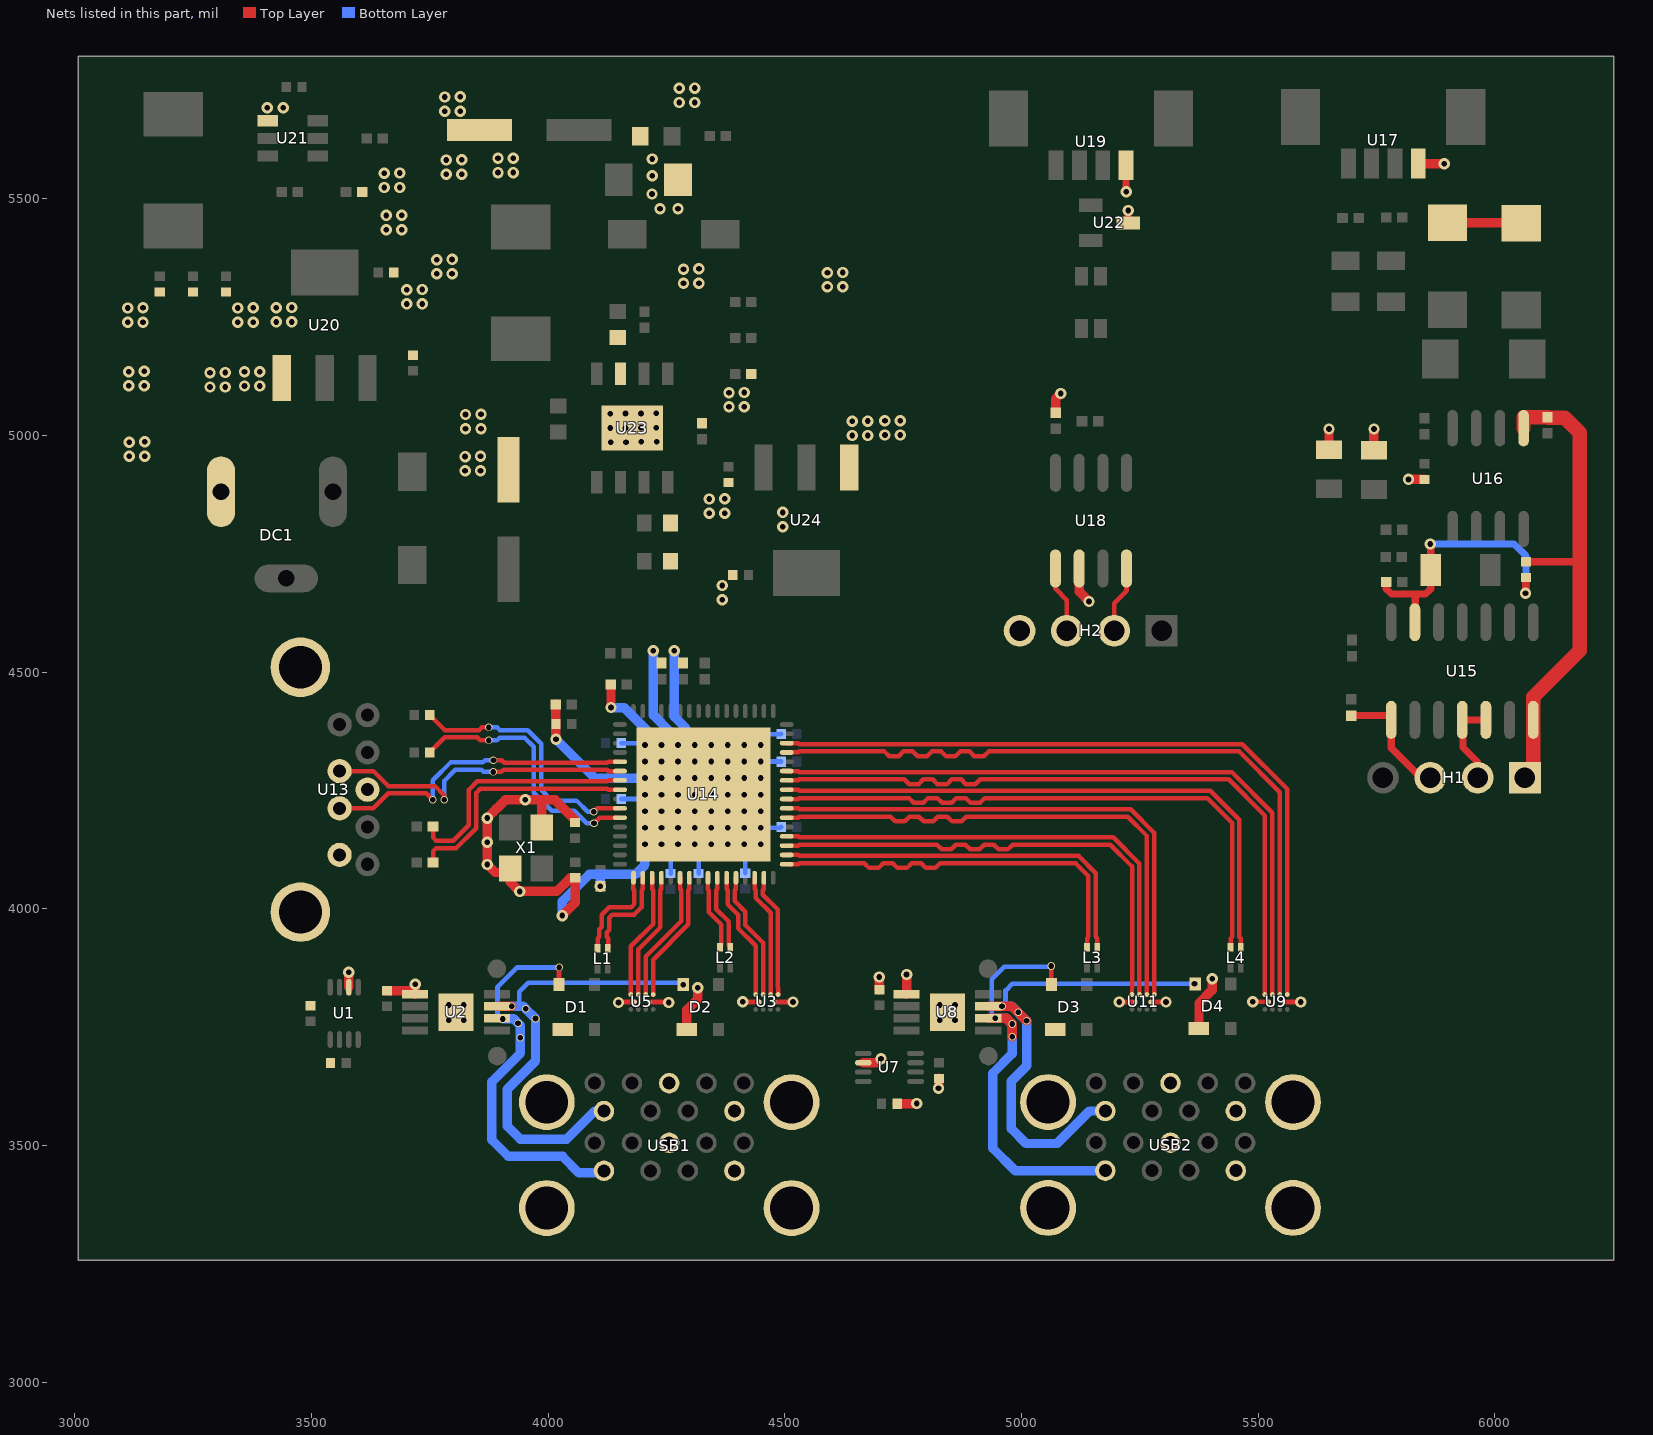
[diagram p0: the nets of this part, all layers, seen from the top]
# Altium PCB MISC51972.pcbdoc (part 3 of 3)
Units mil, origin at the board's own origin, x right, y up, seen from the top; angles counter-clockwise.
Board outline 3243 x 2543 mil, 4 copper layers (Top Layer, GND, Signal-1, Bottom Layer), stack 62.447 mil thick; 117 components, 123 nets, 473 pads, 324 vias.

## Via types
v1: diameter 24.02, hole 12, Top Layer to Bottom Layer, 276 vias
v2: diameter 16, hole 12, Top Layer to Bottom Layer, 47 vias
v3: diameter 24, hole 16, Top Layer to Bottom Layer, 1 vias

## Nets (pads, with @x,y where several pads share a name; then routed paths per layer and width w, separated by ;. In a path a pad name is that pad's centre, name@x,y a point inside that pad or via, vN(x,y) a via of type N, cw(c..) or ccw(c..) an arc to the next point about the centre after c; other vN are vias at no path point) (continued)
GND: C1.1 C2.2 C3.2 C4.1 C5.2 C6.2 C9.1 C10.1 C11.1 C12.1 C13.1 C14.1 C15.2 C16.1 C17.2 C18.1 C19.1 C20.1 C21.1 C23.1 C24.1 C25.1 C27.1 C28.1 C30.1 C31.2 C32.2 C33.1 C34.1 C35.1 C36.1 C37.2 D1.1 D2.1 D3.1 D4.1 DC1.2 H1.1 H2.4 LED1.2 R3.2 R9.2 R11.2 R12.2 R13.2 R16.1 R19.2 R23.2 R27.1 R28.2 RXD1.2 TXD1.2 U1.2 U2.1 U2.9 U3.B1 U3.B2 U5.B1 U5.B2 U7.2 U8.1 U8.9 U9.B1 U9.B2 U11.B1 U11.B2 U13.4 U13.7 U13.10 U14.65 U15.7 U16.5 U17.1 U18.2 U19.1 U20.1 U21.1 U22.3 U23.7 U23.9 U24.1 USB1.4 USB1.7 USB1.13 USB1.16 USB1.19 USB1.20 USB2.4 USB2.7 USB2.13 USB2.16 USB2.19 USB2.20 X1.2 X1.4 | length 4533.2
  Top Layer w10: v1(4148.5,3802.5) 4149.51,3803.51 U5.B1@4182.25,3803.51 ; U5.B2@4213.75,3803.51 4253.49,3803.51 v1(4254.5,3802.5) ; v1(4411,3804) 4411.49,3803.51 U3.B1@4446,3803.51 ; U3.B2@4477.5,3803.51 v1(4517,3803.51) ; v1(5206,3803.51) U11.B1@5241.1,3803.51 ; U11.B2@5272.6,3803.51 v1(5305,3803.51) ; v1(5488.5,3804) 5521.46,3804 U9.B1@5521.95,3803.51 ; U9.B2@5553.45,3803.51 v1(5590,3803.51)
  Top Layer w15: U19.1@5220.66,5571.14 5220.66,5515.34 v1(5221,5515) ; U22.3@5225.01,5449.36 v1(5225,5475.5) ; C21.1@6065.5,4733.54 6178.84,4733.54 6179.1,4733.8
  Top Layer w20: U1.2@3578.64,3834.62 v1(3578.64,3866) ; C2.2@3659.5,3827.54 3710.94,3827.54 U2.1@3718.49,3819.99 3718.49,3840.49 v1(3719,3841) ; X1.2@3986.47,4172.51 3986.47,4228.63 3988.34,4230.5 ; R11.2@4015.76,4432.4 4016.26,4431.9 C17.2@4016.26,4390.72 v1(4016.26,4358.5) ; v1(4029.5,3986) 4057,4013.5 C9.1@4057,4065.76 4046.76,4065.76 4018,4037 v1(3939.5,4037) 3919.53,4056.97 X1.4@3919.53,4085.89 3910.64,4077 3888,4077 v1(3871,4094) v1(3871,4140.97) v1(3871,4192) 3883.63,4204.63 3883.63,4205.16 3890.82,4212.35 3891.35,4212.35 3909.5,4230.5 v1(3951.53,4230.5) 3988.34,4230.5 ; C10.1@4056.7,4182.64 4056.7,4188.3 4014.5,4230.5 3988.34,4230.5 ; R9.2@4132.12,4473.9 4132.5,4473.52 v1(4132.5,4425.5) ; D2.1@4292.87,3745.56 4292.87,3786.87 4316,3810 v1(4316,3833.5) ; U7.2@4665.55,3675.12 4694.62,3675.12 v1(4703,3683.5) ; C5.2@4699.5,3829.54 v1@4699.5,3856.23 ; C6.2@4737.04,3588.5 4778,3588.5 v1(4778.5,3589) ; U8.1@4756.39,3819.99 4756.98,3820.58 v1(4756.98,3861.62) ; v1(4824.5,3621.5) 4825.5,3622.5 C4.1@4825.5,3641.96 ; R19.2@5072.14,5048.44 5072.14,5078.14 v1(5083,5089) ; U18.2@5121.64,4719.18 5121.64,4670.36 v1(5142.5,4649.5) ; D4.1@5374.77,3747.06 5374.77,3800.77 5402.5,3828.5 v1(5402.5,3852.5) ; TXD1.2@5649.45,4970.52 v1(5649.45,5014) ; RXD1.2@5744.45,4969.02 v1(5744.45,5014) ; v1(5817.5,4907.46) C15.2@5851,4907.46 ; U17.1@5837.97,5574.64 v1(5893,5574.64)
  Top Layer w30: U16.5@6060.45,5015.66 6060.45,5038.66 R16.1@6111.45,5038.66 6112.51,5037.6 6147.6,5037.6 6179.1,5006.1 6179.1,4733.8 6179.1,4546.1 6080.95,4447.95 U15.7@6080.95,4399.55 6080.95,4294.95 H1.1@6063.5,4277.5
  Bottom Layer w10: C12.1@4153.94,4232.3 4195.01,4232.3 v1(4204.21,4241.5) ; C20.1@4153.94,4350.3 4200.41,4350.3 v1(4204.21,4346.5) ; C11.1@4258.6,4075.04 4258.6,4120.89 v1(4274.21,4136.5) ; v1(4309.21,4136.5) 4317.8,4127.91 C19.1@4317.8,4075.04 ; v1(4414.21,4136.5) 4416.1,4134.61 C13.1@4416.1,4075.74 ; v1(4449.21,4171.5) 4490.32,4171.5 C14.1@4492.02,4173.2 ; v1(4449.21,4311.5) 4491.52,4311.5 C18.1@4492.02,4311 ; v1(4449.21,4346.5) 4449.21,4362.49 4455.92,4369.21 4491.13,4369.21 C16.1@4492.02,4370.1
  Bottom Layer w20: v1(4016.26,4358.5) 4098.26,4276.5 v1(4204.21,4276.5) ; v1(4029.5,3986) 4029.5,4016 4086.5,4073 4107.62,4073 ; v1(4110,4047.96) 4110,4070.62 4107.62,4073 ; v1(4132.5,4425.5) 4160.21,4425.5 v1(4239.21,4346.5) ; v1(4204.21,4136.5) 4204.21,4093.21 4184,4073 4107.62,4073 ; v1(4222,4545.5) 4222,4409.5 4256.5,4375 ; v1(4266.22,4545.5) 4266.22,4406.28 4290.5,4382
  other v1: 3789.5,3765 3821.5,3765 4827.4,3765 4859.4,3765 3789.5,3797 3821.5,3797 4827.4,3797 4859.4,3797 4699.46,3856.27 4239.21,4136.5 4344.21,4136.5 4379.21,4136.5 4449.21,4136.5 4204.21,4171.5 4239.21,4171.5 4274.21,4171.5 4309.21,4171.5 4344.21,4171.5 4379.21,4171.5 4414.21,4171.5 4204.21,4206.5 4239.21,4206.5 4274.21,4206.5 4309.21,4206.5 4344.21,4206.5 4379.21,4206.5 4414.21,4206.5 4449.21,4206.5 4239.21,4241.5 4274.21,4241.5 4309.21,4241.5 4344.21,4241.5 4379.21,4241.5 4414.21,4241.5 4449.21,4241.5 4239.21,4276.5 4274.21,4276.5 4309.21,4276.5 4344.21,4276.5 4379.21,4276.5 4414.21,4276.5 4449.21,4276.5 4204.21,4311.5 4239.21,4311.5 4274.21,4311.5 4309.21,4311.5 4344.21,4311.5 4379.21,4311.5 4414.21,4311.5 4274.21,4346.5 4309.21,4346.5 4344.21,4346.5 4379.21,4346.5 4414.21,4346.5 4367.25,4653.25 4367.25,4683.25 4495.25,4807.75 4340.25,4836.25 4372.75,4836.25 4495.25,4837.75 4340.25,4866.25 4372.75,4866.75 3824.25,4925.75 3856.75,4925.75 3114.75,4956.25 3147.25,4956.25 3824.25,4955.75 3856.75,4956.25 3114.75,4986.25 4131.75,4986.25 4164.25,4986.25 3147.25,4986.75 4196.75,4986.75 4229.25,4986.75 4642.25,5000.25 4674.75,5000.25 4711.25,5001.25 4743.75,5001.25 3825.25,5014.75 3857.75,5014.75 4130.75,5016.25 4163.25,5016.25 4195.75,5016.75 4228.25,5016.75 4642.25,5030.25 4674.75,5030.75 4711.25,5031.25 4743.75,5031.75 3825.25,5044.75 3857.75,5045.25 4130.75,5046.25 4163.25,5046.75 4195.75,5046.75 4228.25,5047.25 4381.75,5060.75 4414.25,5060.75 4381.75,5090.75 4414.25,5091.25 3285.25,5102.75 3317.75,5102.75 3113.75,5105.25 3146.25,5105.25 3358.25,5104.75 3390.75,5104.75 3285.25,5132.75 3317.75,5133.25 3113.75,5135.25 3358.25,5134.75 3390.75,5135.25 3146.25,5135.75 3111.25,5239.75 3143.75,5239.75 3344.25,5239.75 3376.75,5239.75 3425.25,5240.25 3457.75,5240.25 3111.25,5269.75 3143.75,5270.25 3344.25,5269.75 3376.75,5270.25 3425.25,5270.25 3457.75,5270.75 3701.25,5278.25 3733.75,5278.25 3701.25,5308.25 3733.75,5308.75 4589.75,5314.25 4622.25,5314.25 4285.75,5321.75 4318.25,5321.75 3764.25,5341.75 3796.75,5341.75 4589.75,5344.25 4622.25,5344.75 4285.75,5351.75 4318.25,5352.25 3764.25,5371.75 3796.75,5372.25 3657.75,5435.25 3690.25,5435.25 3657.75,5465.25 3690.25,5465.75 4235.91,5478.99 4274.2,5478.99 4219,5510.5 3653.75,5524.25 3686.25,5524.25 4219.5,5549 3784.75,5552.25 3817.25,5552.25 3653.75,5554.25 3686.25,5554.75 3893.75,5555.75 3926.25,5555.75 3784.75,5582.25 3817.25,5582.75 4219.5,5584.5 3893.75,5585.75 3926.25,5586.25 3781.5,5685.5 3814,5685.5 3406.51,5693 3439.87,5693 4276.75,5703.75 4309.25,5703.75 3781.5,5715.5 3814,5716 4276.75,5733.75 4309.25,5734.25
GND485: D5.2 D7.1 | length 156.2
  Top Layer w20: D7.1@5899.45,5449.39 6054.95,5449.39 D5.2@6055.45,5448.89
P74_TXD6: H1.3 R5.1 U15.1 | length 256.4
  Top Layer w15: R5.1@5696.45,4408.62 5771.88,4408.62 U15.1@5780.95,4399.55 5780.95,4339.75 5843.2,4277.5 H1.3@5863.5,4277.5
P75_RXD6: H1.2 U15.4 U15.5 | length 185.5
  Top Layer w15: H1.2@5963.5,4277.5 5963.5,4310.2 5932.6,4341.1 5932.6,4397.9 U15.4@5930.95,4399.55 U15.5@5980.95,4399.55
P84_CAN_TX2: H2.3 U18.1 | length 141.3
  Top Layer w10: U18.1@5071.64,4719.18 5071.64,4676.36 5095.5,4652.5 5095.5,4588 H2.3@5095.64,4587.86
P85_CAN_RX2: H2.2 U18.4 | length 142.2
  Top Layer w10: H2.2@5195.64,4587.86 5195.5,4588 5195.5,4646 5221.64,4672.14 U18.4@5221.64,4719.18
R5+: C21.2 D8.2 R15.2 U15.13 | length 599.3
  Top Layer w15: R15.2@5770.45,4691.16 5770.45,4676.25 5781.6,4665.1 5831.6,4665.1 ; U15.13@5830.95,4605.77 5831.6,4606.42 5831.6,4665.1 ; v1(5863.1,4771.1) 5864.46,4769.74 D8.2@5864.46,4716.16 5864.46,4675.96 5853.6,4665.1 5831.6,4665.1 ; v1(6064.6,4667.1) 6064.6,4699.56 C21.2@6065.5,4700.46
  Bottom Layer w15: v1(5863.1,4771.1) 6040.6,4771.1 6065.6,4746.1 6065.6,4668.1 v1(6064.6,4667.1)
USB5_5V: D2.4 U2.7 USB1.10 | length 973.4
  Top Layer w20: U2.7@3891.71,3794.4 3891.81,3794.5 v2(3922.5,3794.5)
  Bottom Layer w10: 3936.65,3794.5 3938.5,3796.35 3938.5,3825 3957.5,3844 4281.04,3844 v2(4285,3840.04)
  Bottom Layer w20: v2(3922.5,3794.5) 3936.65,3794.5 3947.5,3794.5 3952.42,3789.58 v2(3952.42,3788.99) v2(3973,3768.41) 3973,3679 3913.5,3619.5 3913.5,3541 3941,3513.5 4038.5,3513.5 4098.13,3573.13 USB1.10@4119,3573.13
USB6_5V: D1.4 U2.6 USB1.1 | length 835.3
  Top Layer w10: D1.4@4022.6,3840.04 4022.6,3876.1 v2(4023,3876.5)
  Bottom Layer w10: v2(3903.5,3767.58) 3892.5,3778.58 3892.5,3834.5 3934.5,3876.5 v2(4023,3876.5)
  Bottom Layer w20: v2(3903.5,3767.58) 3927.28,3767.58 v2(3936.18,3758.68) 3940.68,3754.18 v2(3940.68,3727.99) 3940.68,3694.68 3880.5,3634.5 3880.5,3512.5 3915.5,3477.5 4030.5,3477.5 4030.5,3476.5 4064.5,3442.5 4114.35,3442.5 USB1.1@4119,3447.15
USB7_5V: D4.4 U8.7 USB2.10 | length 1081.4
  Top Layer w20: U8.7@4929.61,3794.4 v2(4958.65,3794.4) 4979.1,3794.4 4991.61,3781.89 v2(4993.11,3781.89) 4993.11,3780.89 v2(5010.5,3763.5)
  Bottom Layer w10: v2(4958.65,3794.4) 4966,3801.75 4966,3827.5 4980.54,3842.04 v2(5365.4,3842.04)
  Bottom Layer w20: v2(4958.65,3794.4) 4979.6,3794.4 v2(5010.5,3763.5) 5010.5,3668.5 4978.5,3636.5 4978.5,3535.5 5009.5,3504.5 5075,3504.5 5143.63,3573.13 USB2.10@5176.88,3573.13
USB8_5V: D3.4 U8.6 USB2.1 | length 922.5
  Top Layer w10: D3.4@5062.9,3840.04 v2(5062.9,3879.5)
  Top Layer w20: U8.6@4929.61,3768.8 v2(4944.33,3768.8) 4968.2,3768.8 v2(4980,3757) v2(4980,3730)
  Bottom Layer w10: v2(4944.33,3768.8) 4937,3776.13 4937,3851.5 4963.5,3878 5061.4,3878 v2(5062.9,3879.5)
  Bottom Layer w20: v2(4944.33,3768.8) 4968.2,3768.8 v2(4980,3757) v2(4980,3730) 4980,3694 4939,3653 4939,3494.5 4986.35,3447.15 USB2.1@5176.88,3447.15
USB30_SSRXM: R2.2 U14.56 | length 517.9
  Top Layer w9.5: R2.2@3756.49,4098.28 3756.49,4121.92 3763.21,4128.63 3805.92,4128.63 3847.5,4170.21 3847.5,4245 3856.53,4254.03 4125.05,4254.03 4127.15,4251.94 U14.56@4151.41,4251.94
USB30_SSRXP: R1.2 U14.55 | length 517.9
  Top Layer w9.5: R1.2@3756.49,4174.48 3756.49,4150.85 3763.21,4144.13 3799.5,4144.13 3832,4176.63 3832,4251.42 3850.11,4269.53 4125.05,4269.53 4127.15,4271.63 U14.55@4151.41,4271.63
USB30_SSTXM: C8.2 U14.59 | length 556.7
  Top Layer w9.5: C8.2@3749.79,4330.78 3781.49,4362.48 3850.1,4362.48 3856.5,4356.09 v2(3874,4356.09) ; v2(4096.63,4181.02) 4108.61,4193 4151.3,4193 U14.59@4151.41,4192.89
  Bottom Layer w9.5: v2(3874,4356.09) 3891.5,4356.09 3897.46,4362.04 3949.96,4362.04 3969.5,4342.5 3969.5,4245.5 4007.5,4207.5 4055.03,4207.5 4081.5,4181.02 v2(4096.63,4181.02)
USB30_SSTXP: C7.2 U14.58 | length 550.8
  Top Layer w9.5: C7.2@3749.79,4409.68 3781.49,4377.98 3853.98,4377.98 3859.5,4383.5 v2(3874.5,4383.5) ; v2(4096.13,4205.16) 4103.54,4212.57 U14.58@4151.41,4212.57
  Bottom Layer w9.5: v2(3874.5,4383.5) 3892,4383.5 3897.96,4377.54 3956.38,4377.54 3985,4348.92 3985,4251.92 4007.92,4229 4059.5,4229 4083.34,4205.16 v2(4096.13,4205.16)
USB30_T_DM1: L1.1 U14.2 | length 206.8
  Top Layer w9.5: L1.1@4126.43,3919.05 4126.43,3937.7 4123.35,3940.78 4123.35,3950.28 4128.78,3955.72 4128.78,3981.57 4135.5,3988.28 4181.75,3988.28 4197.55,4004.08 4197.55,4039.56 4199.64,4041.66 U14.2@4199.64,4065.92
USB30_T_DM2: L2.1 U14.10 | length 159.9
  Top Layer w9.5: U14.10@4357.12,4065.92 4357.12,4041.66 4355.02,4039.56 4355.02,3999.4 4381,3973.42 4381,3922.38 L2.1@4384.33,3919.05
USB30_T_DM3: L3.1 U14.18 | length 826.9
  Top Layer w9.5: U14.18@4503.77,4114.15 4528.03,4114.15 4530.13,4112.06 5120.44,4112.06 5156.75,4075.75 5156.75,3940.78 5159.83,3937.7 L3.1@5159.83,3919.05
USB30_T_DM4: L4.1 U14.25 | length 1253.3
  Top Layer w9.5: U14.25@4503.77,4251.94 4528.03,4251.94 4530.12,4249.85 5398.72,4249.85 5460.15,4188.42 5460.15,3940.78 5463.23,3937.7 L4.1@5463.23,3919.05
USB30_T_DP1: L1.4 U14.1 | length 206.8
  Top Layer w9.5: L1.4@4104.77,3919.05 4104.77,3937.7 4107.85,3940.78 4107.85,3956.7 4113.28,3962.14 4113.28,3987.99 4129.08,4003.78 4175.33,4003.78 4182.05,4010.5 4182.05,4039.56 4179.95,4041.66 U14.1@4179.95,4065.92
USB30_T_DP2: L2.4 U14.9 | length 159.7
  Top Layer w9.5: U14.9@4337.43,4065.92 4337.43,4041.66 4339.52,4039.56 4339.52,3992.97 4365.5,3967 4365.5,3921.88 L2.4@4362.67,3919.05
USB30_T_DP3: L3.4 U14.17 | length 826
  Top Layer w9.5: U14.17@4503.77,4094.46 4528.03,4094.46 4530.13,4096.56 4667.71,4096.56 4677.71,4086.55 4697.71,4086.55 4707.71,4096.56 4727.71,4096.56 4737.71,4086.55 4757.71,4086.55 4767.71,4096.56 4787.71,4096.56 4797.71,4086.55 4817.71,4086.55 4827.71,4096.56 5114.02,4096.56 5141.25,4069.33 5141.25,3940.78 5138.17,3937.7 L3.4@5138.17,3919.05
USB30_T_DP4: L4.4 U14.24 | length 1252.5
  Top Layer w9.5: U14.24@4503.77,4232.26 4528.03,4232.26 4530.12,4234.35 4762.11,4234.35 4772.11,4224.35 4792.11,4224.35 4802.11,4234.35 4822.11,4234.35 4832.11,4224.35 4852.11,4224.35 4862.11,4234.35 4882.11,4234.35 4892.11,4224.35 4912.11,4224.35 4922.11,4234.35 5392.3,4234.35 5444.65,4182 5444.65,3940.78 5441.57,3937.7 L4.4@5441.57,3919.05
USB30_T_SSRXM1: U5.A4 U14.7 | length 278.4
  Top Layer w9.5: U5.A4@4221.62,3819.26 4221.62,3833.76 4221.49,3833.89 4221.49,3892.99 4295.97,3967.47 4295.97,4039.57 4298.06,4041.66 U14.7@4298.06,4065.92
USB30_T_SSRXM2: U3.A4 U14.15 | length 260.7
  Top Layer w9.5: U14.15@4455.54,4065.92 4455.54,4041.66 4453.45,4039.57 4453.45,4030.07 4485.24,3998.27 4485.24,3833.89 4485.37,3833.76 U3.A4@4485.37,3819.26
USB30_T_SSRXM3: U11.A4 U14.23 | length 1139.5
  Top Layer w9.5: U14.23@4503.77,4212.57 4528.03,4212.57 4530.12,4210.48 5230.52,4210.48 5280.35,4160.65 5280.35,3833.89 5280.47,3833.76 U11.A4@5280.47,3819.26
USB30_T_SSRXM4: U9.A4 U14.30 | length 1541
  Top Layer w9.5: U9.A4@5561.32,3819.26 5561.32,3833.76 5561.19,3833.89 5561.19,4253.31 5466.23,4348.27 4530.13,4348.27 4528.03,4350.37 U14.30@4510.19,4350.37 ; U14.30@4510.19,4350.37 U14.30@4503.77,4350.37 4504.8,4349.34 4511.22,4349.34 U14.30@4510.19,4350.37
USB30_T_SSRXP1: U5.A3 U14.6 | length 278.4
  Top Layer w9.5: U5.A3@4205.87,3819.26 4205.87,3833.76 4205.99,3833.89 4205.99,3899.42 4280.47,3973.89 4280.47,4039.57 4278.38,4041.66 U14.6@4278.38,4065.92
USB30_T_SSRXP2: U3.A3 U14.14 | length 260.7
  Top Layer w9.5: U14.14@4435.86,4065.92 4435.86,4041.66 4437.95,4039.57 4437.95,4023.65 4469.74,3991.85 4469.74,3833.89 4469.62,3833.76 U3.A3@4469.62,3819.26
USB30_T_SSRXP3: U11.A3 U14.22 | length 1138.7
  Top Layer w9.5: U14.22@4503.77,4192.89 4528.03,4192.89 4530.12,4194.98 4723.03,4194.98 4733.03,4184.98 4753.03,4184.98 4763.03,4194.98 4783.03,4194.98 4793.03,4184.98 4813.03,4184.98 4823.03,4194.98 4843.03,4194.98 4853.03,4184.98 4873.03,4184.98 4883.03,4194.98 5224.1,4194.98 5264.85,4154.23 5264.85,3833.89 5264.72,3833.76 U11.A3@5264.72,3819.26
USB30_T_SSRXP4: U9.A3 U14.29 | length 1539.2
  Top Layer w9.5: U14.29@4503.77,4330.68 4528.03,4330.68 4530.13,4332.77 4710.28,4332.77 4720.28,4322.77 4740.28,4322.77 4750.28,4332.77 4770.28,4332.77 4780.28,4322.77 4800.28,4322.77 4810.28,4332.77 4830.28,4332.77 4840.28,4322.77 4860.28,4322.77 4870.28,4332.77 4890.28,4332.77 4900.28,4322.77 4920.28,4322.77 4930.28,4332.77 5459.8,4332.77 5545.69,4246.88 5545.69,3833.89 5545.57,3833.76 U9.A3@5545.57,3819.26
USB30_T_SSTXM1: U5.A2 U14.4 | length 267
  Top Layer w9.5: 4189.96,3849.85 4189.96,3914.54 4236.91,3961.49 4236.91,4039.56 4239.01,4041.66 U14.4@4239.01,4065.92 ; 4190.01,3849.81 4190.01,3833.89 4190.13,3833.76 U5.A2@4190.13,3819.26
USB30_T_SSTXM2: U3.A2 U14.12 | length 272.2
  Top Layer w9.5: U14.12@4396.49,4065.92 4396.49,4041.66 4394.4,4039.56 4394.4,4016 4416.49,3993.91 4416.49,3966 4453.76,3928.73 4453.76,3833.89 4453.88,3833.76 U3.A2@4453.88,3819.26
USB30_T_SSTXM3: U11.A2 U14.20 | length 1045.8
  Top Layer w9.5: U14.20@4503.77,4153.52 4528.03,4153.52 4530.13,4151.43 5193.57,4151.43 5248.85,4096.15 5248.85,3833.89 5248.98,3833.76 U11.A2@5248.98,3819.26
USB30_T_SSTXM4: U9.A2 U14.27 | length 1446.5
  Top Layer w9.5: U14.27@4503.77,4291.31 4528.03,4291.31 4530.12,4289.22 5443.78,4289.22 5529.7,4203.3 5529.7,3833.89 5529.83,3833.76 U9.A2@5529.83,3819.26
USB30_T_SSTXP1: U5.A1 U14.3 | length 267
  Top Layer w9.5: U5.A1@4174.38,3819.26 4174.38,3833.76 4174.51,3833.89 4174.51,3849.81 ; 4174.46,3849.85 4174.46,3920.96 4221.41,3967.91 4221.41,4039.56 4219.32,4041.66 U14.3@4219.32,4065.92
USB30_T_SSTXP2: U3.A1 U14.11 | length 272.2
  Top Layer w9.5: U14.11@4376.8,4065.92 4376.8,4041.66 4378.9,4039.56 4378.9,4009.58 4400.99,3987.49 4400.99,3959.58 4438.26,3922.31 4438.26,3833.89 4438.13,3833.76 U3.A1@4438.13,3819.26
USB30_T_SSTXP3: U11.A1 U14.19 | length 1045
  Top Layer w9.5: U14.19@4503.77,4133.83 4528.03,4133.83 4530.13,4135.93 4821.21,4135.93 4831.21,4125.93 4851.21,4125.93 4861.21,4135.93 4881.21,4135.93 4891.21,4125.93 4911.21,4125.93 4921.21,4135.93 4941.21,4135.93 4951.21,4125.93 4971.21,4125.93 4981.21,4135.93 5187.15,4135.93 5233.35,4089.72 5233.35,3833.89 5233.23,3833.76 U11.A1@5233.23,3819.26
USB30_T_SSTXP4: U9.A1 U14.26 | length 1445.6
  Top Layer w9.5: U14.26@4503.77,4271.63 4528.03,4271.63 4530.12,4273.72 4752.29,4273.72 4762.29,4263.72 4782.29,4263.72 4792.29,4273.72 4812.29,4273.72 4822.29,4263.72 4842.29,4263.72 4852.29,4273.72 4872.29,4273.72 4882.29,4263.72 4902.29,4263.72 4912.29,4273.72 5437.36,4273.72 5514.2,4196.87 5514.2,3833.89 5514.08,3833.76 U9.A1@5514.08,3819.26
USB30_USB_DM: U13.2 U14.54 | length 677.3
  Top Layer w9.5: U13.2@3559.07,4291.36 3630.12,4291.35 3661.74,4259.73 3760.54,4259.73 3780.03,4240.25 v2(3780.03,4230.83) ; v2(3883.5,4289.5) 3901,4289.5 3905.6,4294.1 4124.36,4294.1 4127.15,4291.31 U14.54@4151.41,4291.31
  Bottom Layer w9.5: v2(3780.03,4230.83) 3780.03,4270.35 3803.77,4294.1 3858.4,4294.1 3863,4289.5 v2(3883.5,4289.5)
USB30_USB_DP: U13.3 U14.53 | length 673.3
  Top Layer w9.5: U13.3@3559.07,4212.62 3630.12,4212.61 3661.74,4244.23 3742.38,4244.23 v2(3756.04,4230.57) ; v2(3884.1,4314.19) 3901.6,4314.19 3907.19,4308.6 4124.74,4308.6 4127.15,4311 U14.53@4151.41,4311
  Bottom Layer w9.5: v2(3756.04,4230.57) 3756.04,4272.04 3793.6,4309.6 3862,4309.6 3866.6,4314.19 v2(3884.1,4314.19)
pads on no net: DC1.3 U14.32 U14.33 U14.35 U14.36 U14.37 U14.38 U14.39 U14.41 U14.43 U14.44 U14.46 U14.47 U14.60 U17.5 U17.6 U18.5 U19.5 U19.6

## Polygon pours and split planes (outlines as drawn)
1.8V on Signal-1 (solid, remove dead copper): 3443.5,5314 3443.5,5480.29 3416.72,5507.06 3261.56,5507.06 3226.5,5472 3226.5,3916 3374,3768.5 4918,3768.5 4918,3313 4885.5,3280.5 3183.5,3280.5 3060.5,3403.5 3060.5,5517 3167.5,5624 3603,5624 3613,5614 3613,5302.54 3589.7,5279.24 3478.26,5279.24
GND on Top Layer (solid, remove dead copper, pour order 26): 4768,4454 3622,4454 3622,3281.5 3017.5,3281.5 3017.5,4454 3003.25,4454 3003.25,5801 4768,5801
GND on Bottom Layer (solid, remove dead copper, pour order 32): 4765,4453 3632.5,4453 3632.5,3271.5 3000,3271.5 3000,4453 3007.5,4453 3007.5,5801 4765,5801
D5.0V on Signal-1 (solid, remove dead copper): 4894.5,3913.19 4781.31,3800 3350,3800 3233,3917 3233,4362.5 3296.5,4426 3576,4426 3584.5,4417.5 3584.5,4365 3570.5,4351 3399.5,4351 3357.5,4309 3357.5,3982 3407.5,3932 4625,3932 4675.5,3982.5 4675.5,4725.5 4631.5,4769.5 4373,4769.5 4313.5,4829 4313.5,5616.54 4349.29,5652.33 4520.67,5652.33 4547,5626 4547,4961 4587,4921 4866,4921 4894.5,4892.5
12V on Top Layer (solid, remove dead copper, pour order 0): 3495,4963.5 3548,5016.5 3575.5,5016.5 3583.5,5024.5 3583.5,5166.38 3596.13,5179.01 3654.49,5179.01 3679,5154.5 3747,5154.5 3759.5,5142 3759.5,4877 3746,4863.5 3629.5,4863.5 3614.5,4848.5 3614.5,4790.5 3600.5,4776.5 3519.5,4776.5 3495,4801
$1N10192 on Top Layer (solid, remove dead copper, pour order 2): 3671,4798.5 4102,4798.5 4132,4828.5 4132,4927.66 4139.53,4935.19 4214.31,4935.19 4220.5,4929 4220.5,4662.57 4203.62,4645.69 3666.81,4645.69 3641.5,4671 3641.5,4775.5 3665,4799 3670.5,4799
$1N10194 on Top Layer (solid, remove dead copper, pour order 4): 3841,5251 4102.98,5251 4116.78,5237.2 4116.78,5106.75 4114.03,5103 4047,5103 4042,5098 4042,5047.17 4037.07,5042.23 3962.27,5042.23 3954.5,5050 3954.5,5093 3945,5102.5 3836,5102.5 3824.5,5114 3824.5,5234.5
$1N10186 on Top Layer (solid, remove dead copper, pour order 6): 3996.5,5679.5 4131,5679.5 4138,5672.5 4138,5591.32 4145.8,5583.52 4179.98,5583.52 4182.5,5581 4182.5,5464 4185.5,5461 4211,5461 4214.5,5457.5 4214.5,5393 4210,5388.5 3877,5388.5 3870.5,5395 3870.5,5487 3877,5493.5 3978.5,5493.5 3987,5502 3987,5670
D5.0V on Top Layer (solid, remove dead copper, pour order 8): 4371,5659 4362.5,5650.5 4362.5,5475 4353.5,5466 4314,5466 4307.5,5459.5 4307.5,5390.5 4322,5376 4364.5,5376 4373.5,5367 4373.5,5271.59 4382.12,5262.97 4397.97,5262.97 4407,5272 4407,5303 4417.5,5313.5 4454.5,5313.5 4475.5,5334.5 4475.5,5652.5 4468.5,5659.5 4468,5659
1.1V on Top Layer (solid, remove dead copper, pour order 10): 3147,5494.5 3344.5,5494.5 3356.5,5482.5 3356.5,5336.99 3343.91,5324.4 3148.1,5324.4 3137.5,5335 3137.5,5485
1.1V on Signal-1 (solid, remove dead copper): 3259,5484 3349.99,5484 3383.49,5450.5 3383.49,5166.51 3434.5,5115.5 4045,5115.5 4088,5072.5 4088,4090 4126.5,4051.5 4515,4051.5 4553.5,4090 4553.5,4390.5 4570.5,4407.5 4654.5,4407.5 4671.5,4390.5 4671.5,3990.5 4618.5,3937.5 4029.5,3937.5 3921.5,4045.5 3921.5,4903 3839.5,4985 3286.04,4985 3235.81,5035.22 3235.81,5460.81
3.3V on Top Layer (solid, remove dead copper, pour order 12): 4593,5188.5 4593,5064.5 4757.5,5064.5 4757.5,5188.5
1.8V on Top Layer (solid, remove dead copper, pour order 14): 3489,5152 3489,5028.5 3561.5,5028.5 3561.5,5152
GND on Bottom Layer (solid, remove dead copper, pour order 28): 4185.5,4384 4185.5,4100 4469.5,4100 4469.5,4384
GND on Bottom Layer (solid, remove dead copper, pour order 30): 4185.5,4384 4185.5,4100 4469.5,4100 4469.5,4384
GND on Signal-1 (solid, remove dead copper): 4185.5,4384 4185.5,4100 4469.5,4100 4469.5,4384
3.3V on Signal-1 (solid, remove dead copper): 4483.5,4403 4170.5,4403 4170.5,4105 4113,4105 4113,4580.5 4165,4632.5 4438,4632.5 4460,4654.5 4460,4749.23 4471.77,4761 4620,4761 4629,4752 4629,4426.5 4617,4414.5 4538,4414.5 4538,4084.5 4483.5,4084.5
D5.0V on Top Layer (solid, remove dead copper, pour order 16): 3744.8,3806 3748.52,3802.28 3748.52,3788.02 3744,3783.5 3599,3783.5 3584.5,3769 3584.5,3709 3580.5,3705 3557.5,3705 3552,3710.5 3552,3790.5 3567.5,3806
1.8V on Top Layer (solid, remove dead copper, pour order 18): 3482.27,3770.58 3482.27,3702.5 3544,3702.5 3544,3770.58
1.8V on Top Layer (solid, remove dead copper, pour order 20): 4643.5,3661.5 4643.5,3574.7 4713,3574.7 4713,3661.5
D5.0V on Top Layer (solid, remove dead copper, pour order 22): 4756.5,3684 4808.93,3684 4811.83,3686.9 4837.57,3686.9 4841.33,3683.14 4841.33,3665.33 4838,3662 4800.17,3662 4796.67,3658.5 4796.67,3650.67 4793,3647 4757,3647 4752.5,3651.5 4752.5,3680
D5.0V on Top Layer (solid, remove dead copper, pour order 24): 4603.5,3860.5 4603.5,3796.46 4665.93,3796.46 4665.93,3860.5
GND on Bottom Layer (solid, remove dead copper, pour order 34): 4887.5,5806.5 4887.5,4519.5 5423.5,4519.5 5423.5,5806.5
GND on Bottom Layer (solid, remove dead copper, pour order 36): 5520,5804.5 5520,4183 6232.5,4183 6232.5,5804.5

## Keep-outs
Top Layer:
  region: 3809.5,5399.5 3809.5,5248.21 4071.82,5248.21 4071.82,5399.5
  region: 3076.74,5636.45 3076.74,5485.16 3339.06,5485.16 3339.06,5636.45
  region: 4056.7,4182.64 4057,4182.34 4057,4065.76 4046.76,4065.76 4018,4037 3939.5,4037 3939.5,4048.14 3893.64,4094 3871,4094 3871,4192 3898.5,4219.5 4025.5,4219.5 4056.7,4188.3
Board Outline Layer:
  the board outline again, w10

## Silkscreen, mask and mechanical layers (free items; w line width, h text height)
Top Silkscreen Layer:
  lines w20: 4771.48,5801 4771.48,4482 5520,4482 5520,5797.5
  text "GND" at 5909,5548.5 h50
  text "3v3" at 5562.4,5533.5 h50
  text "G" at 5281.4,5524.5 h50
  text "3v3" at 4951.9,5520 h50
  text "A" at 5725.5,5487.5 h50
  text "L" at 5243,5485.5 h50
  text "B" at 5775.5,5486.5 h50
  text "H" at 5080.5,5482 h50
  text "TTL转RS485" at 6242,5138.5 h120 r90
  text "TTL转CAN" at 5472.5,4948.5 h120 r90
  text "G" at 4979.65,4485.5 h50
  text "RX" at 5066.45,4485.5 h50
  text "TX" at 5166,4486 h50
  text "3v3" at 5251.5,4485.5 h50
  text "3v3" at 5717.5,4173 h50
  text "TX" at 5833,4173 h50
  text "RX" at 5932.4,4173 h50
  text "G" at 6049,4173 h50